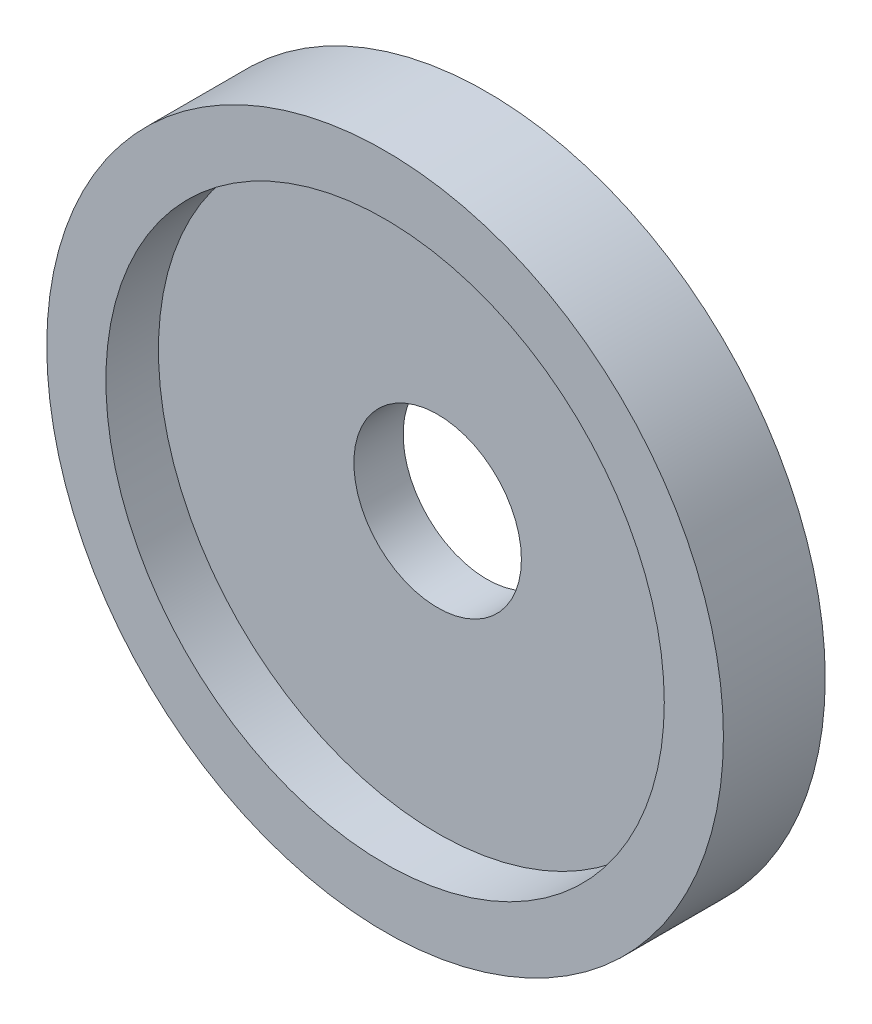
SolidWorks part; units mm, degrees
ref_plane "Front Plane" through (0, 0, 0) normal (0, 0, 1) x (1, 0, 0)
ref_plane "Top Plane" through (0, 0, 0) normal (0, 1, 0) x (1, 0, 0)
ref_plane "Right Plane" through (0, 0, 0) normal (1, 0, 0) x (0, 0, -1)
sketch "Sketch1" plane through (0, 0, 0) normal (0, 0, 1) x (1, 0, 0)
  circle A0 centre (0, 0) radius 103
  circle A1 centre (0, 0) radius 25.5
  dimension "D1" = 206
  dimension "D2" = 51
extrude "Boss-Extrude1" add sketch "Sketch1" along normal blind 15
sketch "Sketch2" plane through (0, 0, 15) normal (0, 0, 1) x (1, 0, 0)
  circle A0 centre (0, 0) radius 85
  circle A1 centre (0, 0) radius 103
  dimension "D1" = 170
  dimension "D2" = 206
extrude "Boss-Extrude2" add sketch "Sketch2" along normal blind 16
